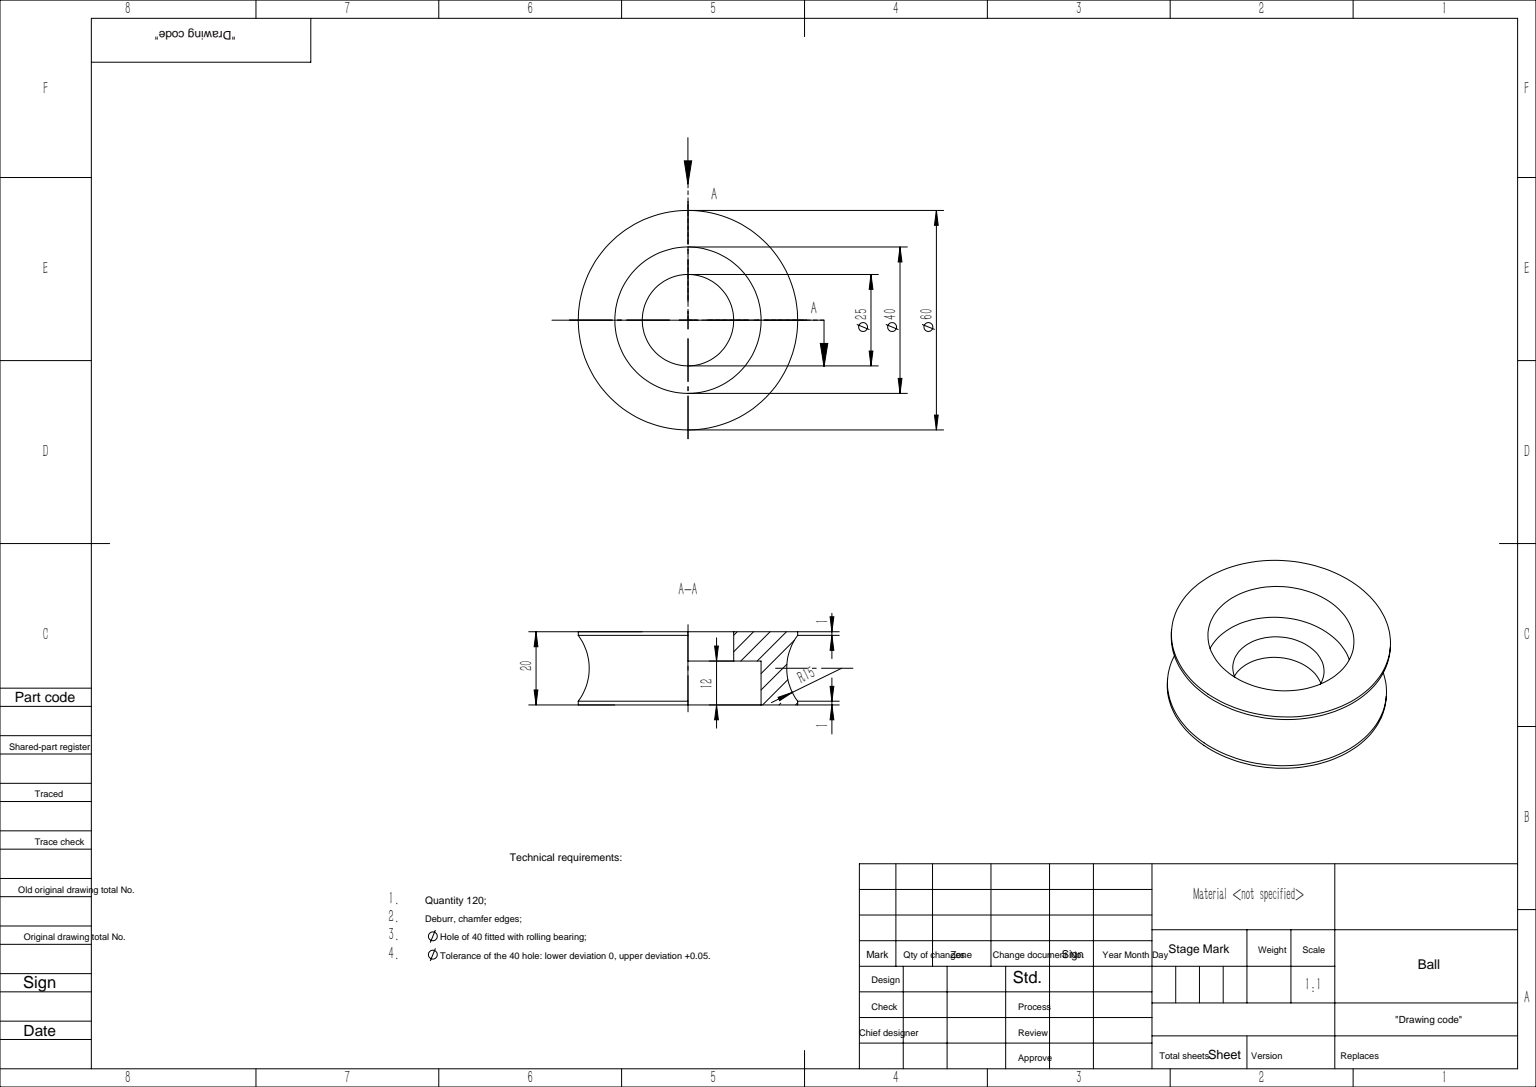
SolidWorks part; units mm, degrees
ref_plane "前视基准面" through (0, 0, 0) normal (0, 0, 1) x (1, 0, 0)
ref_plane "上视基准面" through (0, 0, 0) normal (0, 1, 0) x (1, 0, 0)
ref_plane "右视基准面" through (0, 0, 0) normal (1, 0, 0) x (0, 0, -1)
sketch "草图1" plane through (0, 0, 0) normal (0, 1, 0) x (1, 0, 0)
  circle A0 centre (0, 0) radius 30
  dimension "D1" = 60
extrude "凸台-拉伸1" add sketch "草图1" along normal blind 20
sketch "草图2" plane through (0, 20, 0) normal (0, 1, 0) x (1, 0, 0)
  circle A0 centre (0, 0) radius 20
  dimension "D1" = 40
extrude "切除-拉伸1" cut sketch "草图2" against normal blind 12
sketch "草图4" plane through (0, 8, 0) normal (0, 1, 0) x (1, 0, 0)
  circle A0 centre (0, 0) radius 12.5
  dimension "D1" = 25
extrude "切除-拉伸2" cut sketch "草图4" against normal through all and the other way through all
sketch "草图5" plane through (0, 0, 0) normal (0, 0, 1) x (1, 0, 0)
  line L0 (30, 10) -> (-30, 10) construction
  line L1 (30, 0) -> (30, 20) construction
  line L2 (-30, 20) -> (-30, 0) construction
  line L4 (0, 0) -> (0, 36.1614) construction
  line L5 (-30, 19) -> (30, 19) construction
  line L6 (30, 20) -> (-30, 20) construction
  circle A0 centre (42, 10) radius 15
  dimension "D1" = 30
  dimension "D2" = 1
revolve "切除-旋转1" cut sketch "草图5" angle 360 about L4
